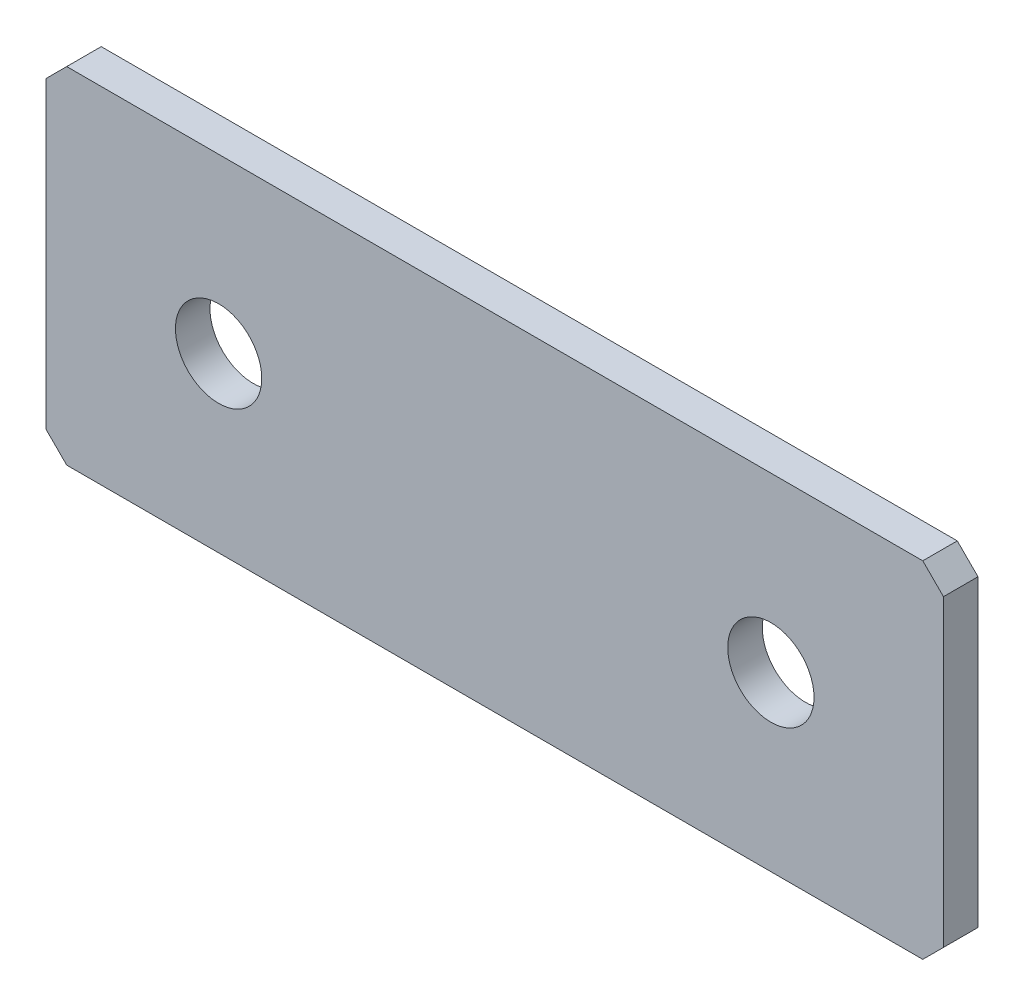
from build123d import *

# Parameters (mm, degrees)
SKETCH1_R           = 6.25
BOSS_EXTRUDE1_DEPTH = 5


with BuildPart() as part:
    # Sketch1 → Boss-Extrude1 (new body)
    with BuildSketch(Plane.XY.offset(2.5)):
        Polygon((-62, -25), (62, -25), (65, -22), (65, 22), (62, 25), (-62, 25), (-65, 22), (-65, -22), align=None)
        with Locations((-40, 0)):
            Circle(SKETCH1_R, mode=Mode.SUBTRACT)
        with Locations((40, 0)):
            Circle(SKETCH1_R, mode=Mode.SUBTRACT)
    extrude(amount=-BOSS_EXTRUDE1_DEPTH)


solid = part.part
